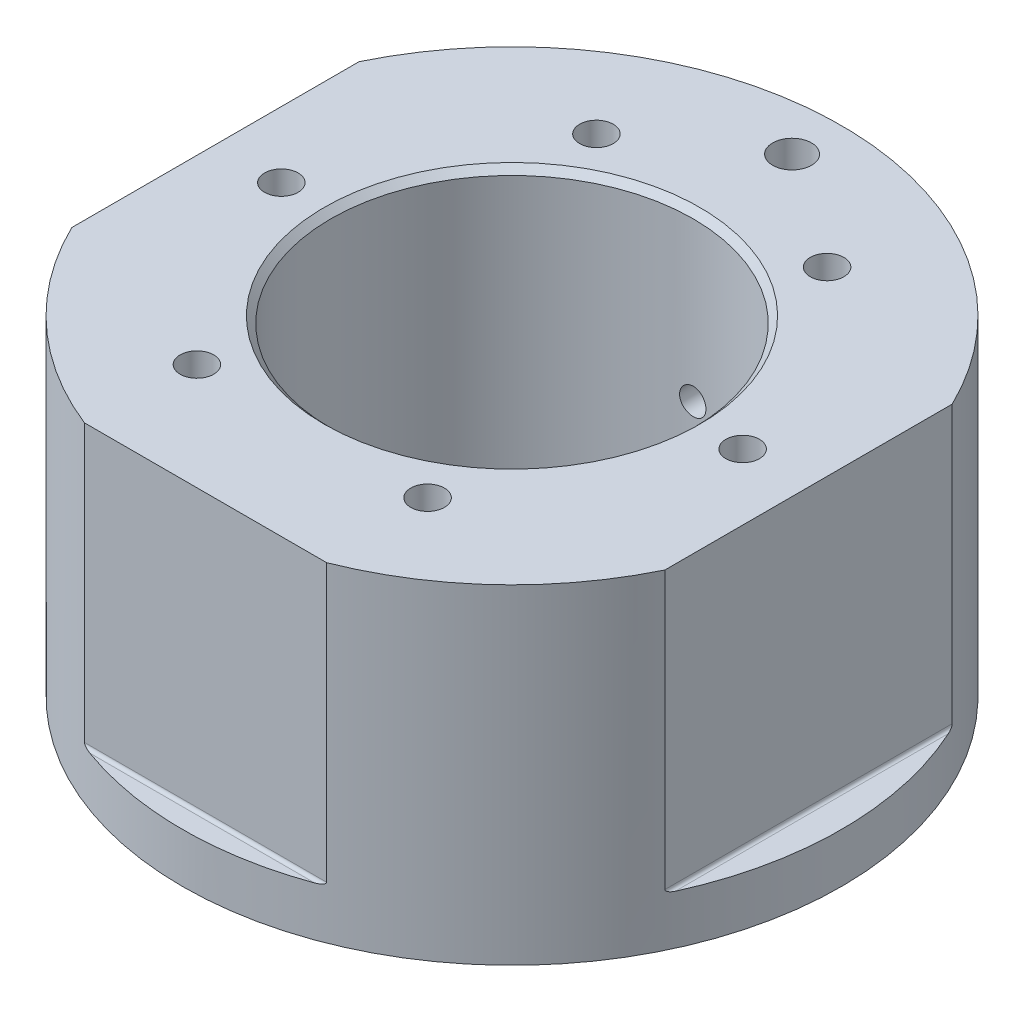
SolidWorks part; units mm, degrees
ref_plane "Front Plane" through (0, 0, 0) normal (0, 0, 1) x (1, 0, 0)
ref_plane "Top Plane" through (0, 0, 0) normal (0, 1, 0) x (1, 0, 0)
ref_plane "Right Plane" through (0, 0, 0) normal (1, 0, 0) x (0, 0, -1)
sketch "Sketch1" plane through (0, 0, 0) normal (0, 1, 0) x (1, 0, 0)
  circle A0 centre (0, 0) radius 100
  dimension "D1" = 200
extrude "Boss-Extrude1" add sketch "Sketch1" along normal blind 100
sketch "Sketch2" plane through (0, 100, 0) normal (0, 1, 0) x (1, 0, 0)
  line L0 (0, 0) -> (0, 126.2792) construction
  line L5 (-36.756, -93) -> (36.756, -93)
  line L6 (-90, -43.589) -> (-90, 43.589)
  line L7 (90, -43.589) -> (90, 43.589)
  arc A1 (-90, 43.589) -> (-90, -43.589) centre (0, 0) ccw
  circle A2 centre (0, 0) radius 100
  arc A3 (-36.756, -93) -> (36.756, -93) centre (0, 0) ccw
  arc A4 (90, -43.589) -> (90, 43.589) centre (0, 0) ccw
  point P8 (0, -93)
  point P11 (-90, 0)
  dimension "D1" = 0
  dimension "D2" = 93
  dimension "D3" = 180
extrude "Cut-Extrude1" cut sketch "Sketch2" against normal blind 85
sketch "Sketch3" plane through (0, 100, 0) normal (0, 1, 0) x (1, 0, 0)
  circle A0 centre (0, 0) radius 55
  dimension "D1" = 110
extrude "Cut-Extrude2" cut sketch "Sketch3" against normal through all
chamfer "Chamfer1" distance 2 angle 45 2 edges at (0, 0, 55) (0, 100, 55)
sketch "Sketch4" plane through (0, 100, 0) normal (0, 1, 0) x (1, 0, 0)
  line L0 (0, 0) -> (0, 83.7409) construction
  line L1 (0, 0) -> (-35, 60.6218) construction
  dimension "D1" = 70
  dimension "D2" = 30
hole_wizard "M12 Tapped Hole1" positions "Sketch5" profile "Sketch6" tap size "M12" standard "GB"
sketch "Sketch5" plane through (0, 100, 0) normal (0, 1, 0) x (1, 0, 0)
  point P0 (-35, 60.6218)
sketch "Sketch6" plane through (-35, 100, -60.6218) normal (1, 0, 0) x (0, 0, 1)
  line L0 (0, 0) -> (0, 38.3144)
  line L1 (0, 38.3144) -> (5.1, 35.25)
  line L2 (5.1, 35.25) -> (5.1, 0)
  line L5 (5.1, 0) -> (0, 0)
  line L10 (0, 38.3144) -> (-5.1, 35.25) construction
  line L11 (0, -6.35) -> (0, 107.95) construction
  dimension "螺纹孔钻头直径" = 10.2
  dimension "螺纹孔钻头深度" = 35.25
  dimension "导头角度" = 118
cosmetic thread "Cosmetic Thread1"
sketch "Sketch7" plane through (0, 0, 0) normal (0, -1, 0) x (1, 0, 0)
  point P0 (-35, -60.6218)
hole_wizard "M12 Tapped Hole2" positions "Sketch8" profile "Sketch9" tap size "M12" standard "GB"
sketch "Sketch8" plane through (0, 0, 0) normal (0, -1, 0) x (-1, 0, 0)
  point P0 (35, 60.6218)
sketch "Sketch9" plane through (-35, 0, -60.6218) normal (1, 0, 0) x (0, 0, -1)
  line L0 (0, 0) -> (0, 38.3144)
  line L1 (0, 38.3144) -> (5.1, 35.25)
  line L2 (5.1, 35.25) -> (5.1, 0)
  line L5 (5.1, 0) -> (0, 0)
  line L10 (0, 38.3144) -> (-5.1, 35.25) construction
  line L11 (0, -6.35) -> (0, 107.95) construction
  dimension "螺纹孔钻头直径" = 10.2
  dimension "螺纹孔钻头深度" = 35.25
  dimension "导头角度" = 118
cosmetic thread "Cosmetic Thread2"
sketch "Sketch10" plane through (0, 0, 0) normal (0, -1, 0) x (1, 0, 0)
  circle A0 centre (-35, -60.6218) radius 4
  dimension "D1" = 8
extrude "Cut-Extrude3" cut sketch "Sketch10" against normal through all
pattern_circular "CirPattern1" count 6 over 360 about axis through (0, 0, 0) along (0, 1, 0) of "M12 Tapped Hole1", "M12 Tapped Hole2", "Cut-Extrude3"
sketch "Sketch11" plane through (0, 100, 0) normal (0, 1, 0) x (1, 0, 0)
  point P0 (0, 85)
  dimension "D1" = 85
hole_wizard "G1/4 Tapped Hole1" positions "Sketch12" profile "Sketch13" tap size "G1/4" standard "GB"
sketch "Sketch12" plane through (0, 100, 0) normal (0, 1, 0) x (1, 0, 0)
  point P0 (0, 85)
sketch "Sketch13" plane through (0, 100, -85) normal (1, 0, 0) x (0, 0, 1)
  line L0 (0, 0) -> (0, 13.5451)
  line L1 (0, 13.5451) -> (5.9, 10)
  line L2 (5.9, 10) -> (5.9, 0)
  line L5 (5.9, 0) -> (0, 0)
  line L10 (0, 13.5451) -> (-5.9, 10) construction
  line L11 (0, -6.35) -> (0, 107.95) construction
  dimension "螺纹孔钻头直径" = 11.8
  dimension "螺纹孔钻头深度" = 10
  dimension "导头角度" = 118
cosmetic thread "Cosmetic Thread3"
hole_wizard "Ø8.0 (8) Diameter Hole1" positions "Sketch14" profile "Sketch15" hole size "Ø8.0" standard "GB"
sketch "Sketch14" plane through (0, 100, 0) normal (0, 1, 0) x (1, 0, 0)
  point P0 (0, 85)
sketch "Sketch15" plane through (0, 100, -85) normal (1, 0, 0) x (0, 0, 1)
  line L0 (0, 0) -> (0, 62.4034)
  line L1 (0, 62.4034) -> (4, 60)
  line L2 (4, 60) -> (4, 0)
  line L5 (4, 0) -> (0, 0)
  line L10 (0, 62.4034) -> (-4, 60) construction
  line L11 (0, -6.35) -> (0, 107.95) construction
  dimension "孔直径" = 8
  dimension "孔深度" = 60
  dimension "导头角度" = 118
hole_wizard "Ø8.0 (8) Diameter Hole2" positions "3DSketch1" profile "Sketch16" hole size "Ø8.0" standard "GB"
sketch3d "3DSketch1"
  line L0 (0, 0, 0) -> (0, 0, -100) construction
  line L1 (0, 0, -100) -> (0, 100, -100) construction
  circle A0 centre (0, 0, 0) radius 100 construction
  arc A1 (90, 100, -43.589) -> (-90, 100, -43.589) centre (0, 100, 0) ccw construction
  point P0 (0, 50, -100)
  point P8 (0, 100, 0)
  point P13 (0, 200, 0)
  dimension "D1" = 50
sketch "Sketch16" plane through (0, 50, -100) normal (1, 0, 0) x (0, 1, 0)
  line L0 (0, 0) -> (0, 62.4034)
  line L1 (0, 62.4034) -> (4, 60)
  line L2 (4, 60) -> (4, 0)
  line L5 (4, 0) -> (0, 0)
  line L10 (0, 62.4034) -> (-4, 60) construction
  line L11 (0, -6.35) -> (0, 107.95) construction
  dimension "孔直径" = 8
  dimension "孔深度" = 60
  dimension "导头角度" = 118
fillet "Fillet1" radius 1 3 edges at (-90, 15, 0) (90, 15, 0) (0, 15, 93)
